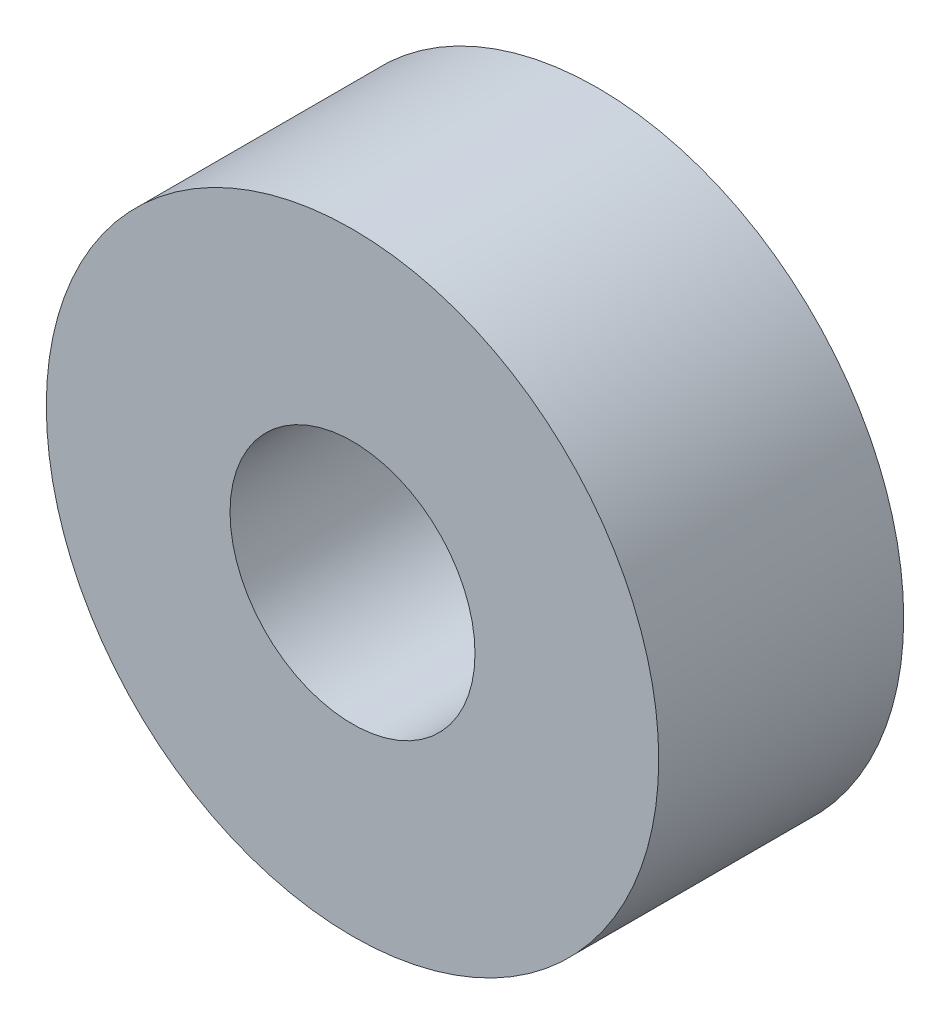
SolidWorks part; units mm, degrees
ref_plane "Front Plane" through (0, 0, 0) normal (0, 0, 1) x (1, 0, 0)
ref_plane "Top Plane" through (0, 0, 0) normal (0, 1, 0) x (1, 0, 0)
ref_plane "Right Plane" through (0, 0, 0) normal (1, 0, 0) x (0, 0, -1)
sketch "Sketch1" plane through (0, 0, 0) normal (0, 0, 1) x (1, 0, 0)
  circle A0 centre (-220.5, 0) radius 2.5
  circle A1 centre (-220.5, 0) radius 1
  dimension "D1" = 2
extrude "Boss-Extrude1" add sketch "Sketch1" along normal blind 2
